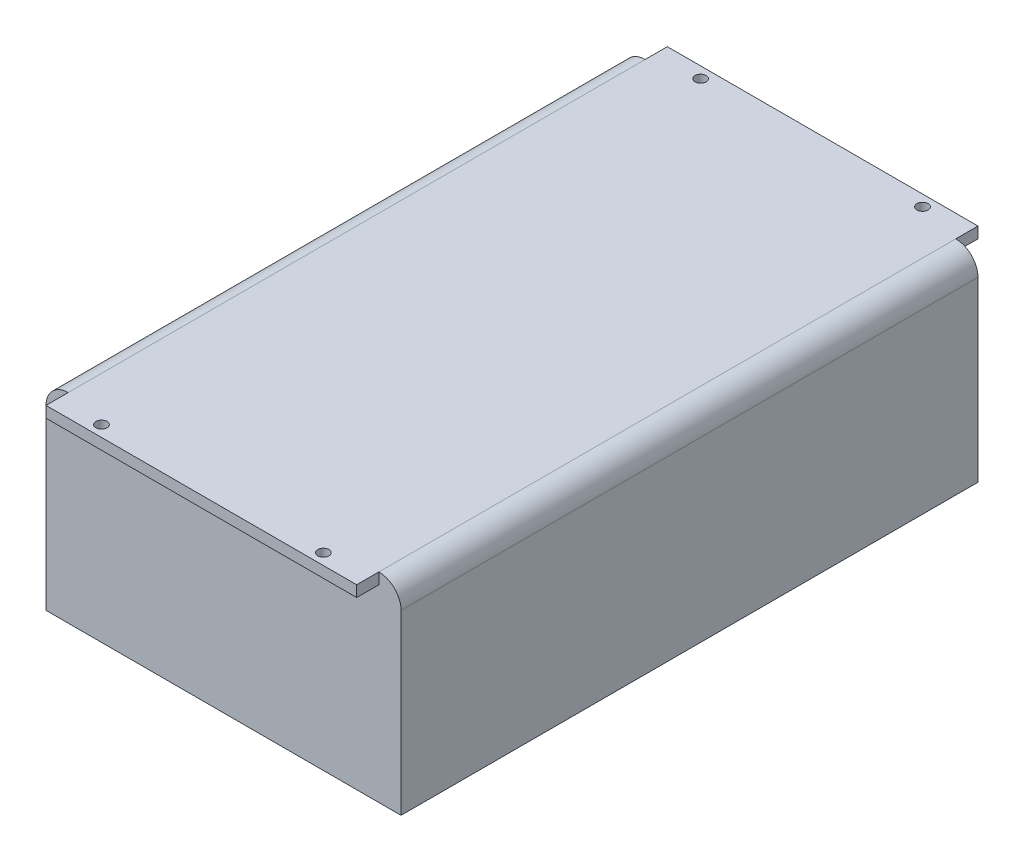
from build123d import *

# Parameters (mm, degrees)
SKETCH1_W           = 160
SKETCH1_H           = 90
BOSS_EXTRUDE1_DEPTH = 260
FILLET2_R           = 10
SHELL1_T            = -3
SKETCH2_R           = 5
SKETCH2_R_2         = 2
BOSS_EXTRUDE2_DEPTH = 50
SKETCH3_R           = 6
SKETCH3_R_2         = 2
BOSS_EXTRUDE3_DEPTH = 6
SKETCH4_W           = 140
SKETCH4_H           = 5
BOSS_EXTRUDE4_DEPTH = 10
SKETCH5_W           = 140
SKETCH5_H           = 5
BOSS_EXTRUDE5_DEPTH = 10
SKETCH6_R           = 2.5
CUT_EXTRUDE1_DEPTH  = 326.153809758


with BuildPart() as part:
    # Sketch1 → Boss-Extrude1 (new body)
    with BuildSketch(Plane.XY):
        with Locations((80, 45)):
            Rectangle(SKETCH1_W, SKETCH1_H)
    extrude(amount=BOSS_EXTRUDE1_DEPTH)

    # Fillet2
    fillet2_edges = [part.edges().sort_by_distance(p)[0] for p in [
        (0, 90, 130),
        (160, 90, 130),
    ]]
    fillet(fillet2_edges, radius=FILLET2_R)

    # Shell1
    shell1_openings = [part.faces().sort_by_distance(p)[0] for p in [
        (80, 0, 130),
    ]]
    offset(amount=SHELL1_T, openings=shell1_openings, kind=Kind.INTERSECTION)

    # Sketch2 → Boss-Extrude2 (add)
    # profile 1 of 4: a face of its own
    with BuildSketch(Plane(origin=(0, 87, 0), x_dir=(-1, 0, 0), z_dir=(0, -1, 0))):
        with Locations(Location((-35, -88.2, 0), (0, 0, 90))):
            Circle(SKETCH2_R)
        with Locations(Location((-35, -88.2, 0), (0, 0, 90))):
            Circle(SKETCH2_R_2, mode=Mode.SUBTRACT)
    # profile 2 of 4: a face of its own
    with BuildSketch(Plane(origin=(0, 87, 0), x_dir=(-1, 0, 0), z_dir=(0, -1, 0))):
        with Locations(Location((-35, -12, 0), (0, 0, 90))):
            Circle(SKETCH2_R)
        with Locations(Location((-35, -12, 0), (0, 0, 90))):
            Circle(SKETCH2_R_2, mode=Mode.SUBTRACT)
    # profile 3 of 4: a face of its own
    with BuildSketch(Plane(origin=(0, 87, 0), x_dir=(-1, 0, 0), z_dir=(0, -1, 0))):
        with Locations(Location((-137.87, -12, 0), (0, 0, 90))):
            Circle(SKETCH2_R)
        with Locations(Location((-137.87, -12, 0), (0, 0, 90))):
            Circle(SKETCH2_R_2, mode=Mode.SUBTRACT)
    # profile 4 of 4: a face of its own
    with BuildSketch(Plane(origin=(0, 87, 0), x_dir=(-1, 0, 0), z_dir=(0, -1, 0))):
        with Locations(Location((-137.87, -88.2, 0), (0, 0, 90))):
            Circle(SKETCH2_R)
        with Locations(Location((-137.87, -88.2, 0), (0, 0, 90))):
            Circle(SKETCH2_R_2, mode=Mode.SUBTRACT)
    extrude(amount=BOSS_EXTRUDE2_DEPTH)

    # Sketch3 → Boss-Extrude3 (add)
    # profile 1 of 4: a face of its own
    with BuildSketch(Plane(origin=(0, 87, 0), x_dir=(-1, 0, 0), z_dir=(0, -1, 0))):
        with Locations(Location((-20, -114, 0), (0, 0, 90))):
            Circle(SKETCH3_R)
        with Locations(Location((-20, -114, 0), (0, 0, 90))):
            Circle(SKETCH3_R_2, mode=Mode.SUBTRACT)
    # profile 2 of 4: a face of its own
    with BuildSketch(Plane(origin=(0, 87, 0), x_dir=(-1, 0, 0), z_dir=(0, -1, 0))):
        with Locations(Location((-20, -250, 0), (0, 0, 90))):
            Circle(SKETCH3_R)
        with Locations(Location((-20, -250, 0), (0, 0, 90))):
            Circle(SKETCH3_R_2, mode=Mode.SUBTRACT)
    # profile 3 of 4: a face of its own
    with BuildSketch(Plane(origin=(0, 87, 0), x_dir=(-1, 0, 0), z_dir=(0, -1, 0))):
        with Locations(Location((-140, -114, 0), (0, 0, 90))):
            Circle(SKETCH3_R)
        with Locations(Location((-140, -114, 0), (0, 0, 90))):
            Circle(SKETCH3_R_2, mode=Mode.SUBTRACT)
    # profile 4 of 4: a face of its own
    with BuildSketch(Plane(origin=(0, 87, 0), x_dir=(-1, 0, 0), z_dir=(0, -1, 0))):
        with Locations(Location((-140, -250, 0), (0, 0, 90))):
            Circle(SKETCH3_R)
        with Locations(Location((-140, -250, 0), (0, 0, 90))):
            Circle(SKETCH3_R_2, mode=Mode.SUBTRACT)
    extrude(amount=BOSS_EXTRUDE3_DEPTH)

    # Sketch4 → Boss-Extrude4 (add)
    with BuildSketch(Plane(origin=(0, 0, 0), x_dir=(-1, 0, 0), z_dir=(0, 0, -1))):
        with Locations((-80, 87.5)):
            Rectangle(SKETCH4_W, SKETCH4_H)
    extrude(amount=BOSS_EXTRUDE4_DEPTH)

    # Sketch5 → Boss-Extrude5 (add)
    with BuildSketch(Plane.XY.offset(260)):
        with Locations((80, 87.5)):
            Rectangle(SKETCH5_W, SKETCH5_H)
    extrude(amount=BOSS_EXTRUDE5_DEPTH)

    # Sketch6 → Cut-Extrude1 (cut, through all)
    with BuildSketch(Plane(origin=(0, 85, 0), x_dir=(-1, 0, 0), z_dir=(0, -1, 0))):
        with Locations(Location((-130, -265, 0), (0, 0, 180))):
            Circle(SKETCH6_R)
        with Locations(Location((-30, -265, 0), (0, 0, 180))):
            Circle(SKETCH6_R)
        with Locations(Location((-130, 5, 0), (0, 0, 180))):
            Circle(SKETCH6_R)
        with Locations(Location((-30, 5, 0), (0, 0, 180))):
            Circle(SKETCH6_R)
    extrude(amount=-CUT_EXTRUDE1_DEPTH, mode=Mode.SUBTRACT)


solid = part.part
